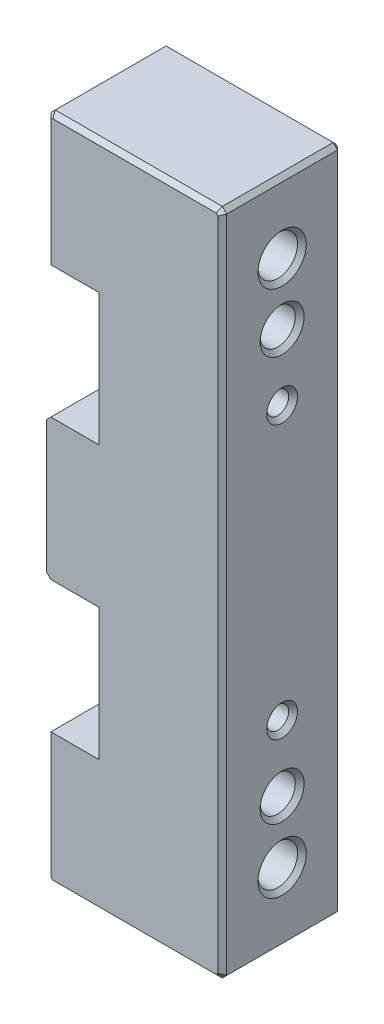
from build123d import *

# Parameters (mm, degrees)
EXTRUDE_1_DEPTH              = 13.6
CHAMFER_1_SIZE               = 0.5
HOLE_WIZARD_M4_1_D           = 4.5
HOLE_WIZARD_M4_1_CBORE_D     = 8
HOLE_WIZARD_M4_1_CBORE_DEPTH = 4.4
SKETCH_6_W                   = 2
SKETCH_6_H                   = 15
EXTRUDE_2_DEPTH              = 13.6
HOLE_WIZARD_M3_1_D           = 2.5
MM_1_D                       = 4
MM_1_DEPTH                   = 10
MM_1_TIP                     = 1.201721238
CHAMFER_2_SIZE               = 0.5
MM_2_D                       = 3
MM_2_DEPTH                   = 1
MM_2_TIP                     = 0.901290929


with BuildPart() as part:
    # 草图3 → 凸台-拉伸1 (new body)
    with BuildSketch(Plane.XY):
        Polygon((10, 37.5), (9.5, 38), (-9.5, 38), (-10, 37.5), (-10, 23.5), (-9.5, 23), (-2, 23), (-2, 8), (-9.5, 8), (-10, 7.5), (-10, -7.5), (-9.5, -8), (-2, -8), (-2, -23), (-9.5, -23), (-10, -23.5), (-10, -37.5), (-9.5, -38), (9.5, -38), (10, -37.5), align=None)
    extrude(amount=-EXTRUDE_1_DEPTH)

    # 倒角1
    chamfer_1_edges = [part.edges().sort_by_distance(p)[0] for p in [
        (-10, 30.5, -13.6),
        (-9.75, 37.75, -13.6),
        (0, 38, -13.6),
        (9.75, 37.75, -13.6),
        (10, 0, -13.6),
        (9.75, -37.75, -13.6),
        (-10, -30.5, -13.6),
        (-9.75, -37.75, -13.6),
        (0, -38, -13.6),
        (-10, 30.5, 0),
        (-9.75, 37.75, 0),
        (0, 38, 0),
        (9.75, 37.75, 0),
        (10, 0, 0),
        (9.75, -37.75, 0),
        (-10, -30.5, 0),
        (-9.75, -37.75, 0),
        (0, -38, 0),
    ]]
    chamfer(chamfer_1_edges, length=CHAMFER_1_SIZE)

    # M4 六角凹头螺钉的柱形沉头孔1 (through all)
    with Locations(Plane.ZY.offset(10)):
        with Locations((-6.8, -30), (-6.8, 30)):
            CounterBoreHole(HOLE_WIZARD_M4_1_D / 2, HOLE_WIZARD_M4_1_CBORE_D / 2, HOLE_WIZARD_M4_1_CBORE_DEPTH)

    # 草图6 → 凸台-拉伸2 (add)
    with BuildSketch(Plane.XY):
        with Locations((-3, -15.5)):
            Rectangle(SKETCH_6_W, SKETCH_6_H)
        with Locations((-3, 15.5)):
            Rectangle(SKETCH_6_W, SKETCH_6_H)
    extrude(amount=-EXTRUDE_2_DEPTH)

    # M3 螺纹孔1 (through all)
    with Locations(Plane.ZY.offset(4)):
        with Locations((-6.8, -15.5), (-6.8, 15.5)):
            Hole(HOLE_WIZARD_M3_1_D / 2)

    # 大小mm 暗销孔1
    with Locations(Plane(origin=(10, 0, 0), x_dir=(0, 0, -1), z_dir=(1, 0, 0))):
        with Locations((6.8, -23), (6.8, 23)):
            Hole(MM_1_D / 2, depth=MM_1_DEPTH)
            with Locations((0, 0, -(MM_1_DEPTH + MM_1_TIP / 2))):  # 118° drill point
                Cone(0, MM_1_D / 2, MM_1_TIP, mode=Mode.SUBTRACT)

    # 倒角2
    chamfer_2_edges = [part.edges().sort_by_distance(p)[0] for p in [
        (-10, 30, -10.8),
        (10, 30, -4.55),
        (-10, -30, -10.8),
        (10, -30, -4.55),
        (10, 15.5, -5.55),
        (10, -15.5, -5.55),
        (10, 23, -8.8),
        (10, -23, -8.8),
    ]]
    chamfer(chamfer_2_edges, length=CHAMFER_2_SIZE)

    # 大小mm 暗销孔2
    with Locations(Plane.ZY.offset(10)):
        with Locations((-6.8, 0)):
            Hole(MM_2_D / 2, depth=MM_2_DEPTH)
            with Locations((0, 0, -(MM_2_DEPTH + MM_2_TIP / 2))):  # 118° drill point
                Cone(0, MM_2_D / 2, MM_2_TIP, mode=Mode.SUBTRACT)


solid = part.part
